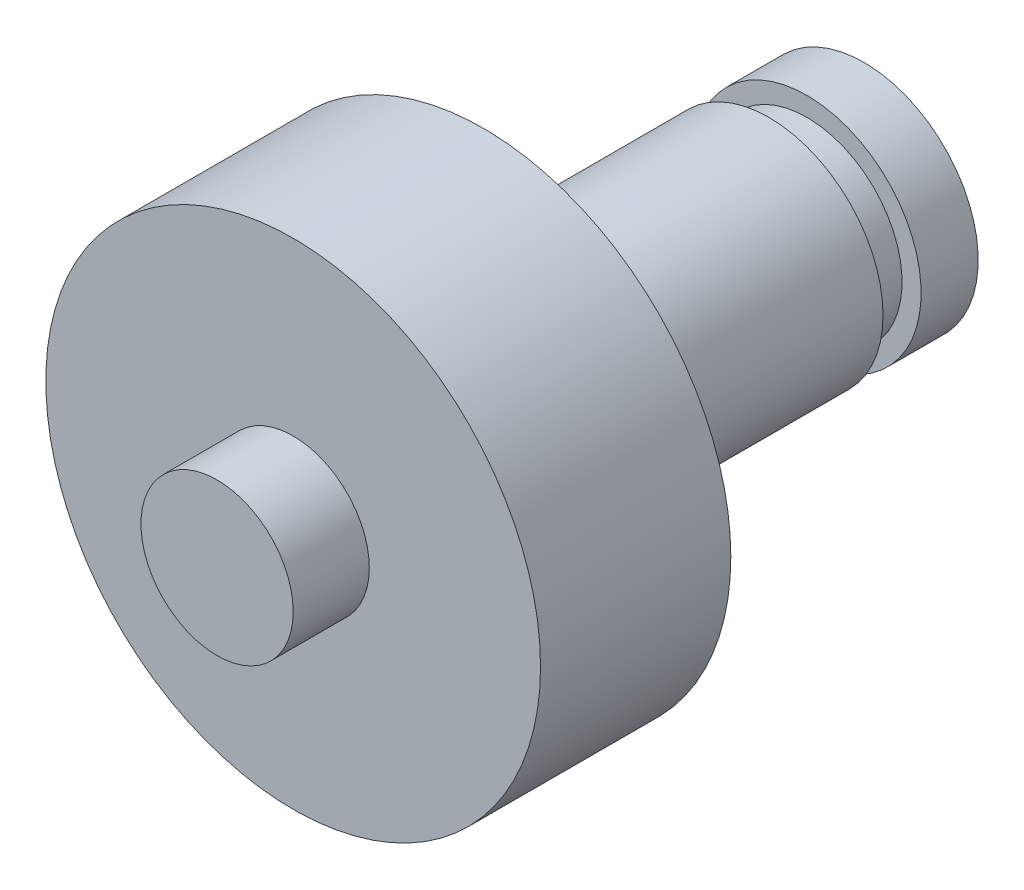
from build123d import *

# Parameters (mm, degrees)
SKETCH1_R      = 6.5
EXTRUDE1_DEPTH = 5
SKETCH2_R      = 2
EXTRUDE2_DEPTH = 2
SKETCH3_R      = 3
EXTRUDE3_DEPTH = 7.5
SKETCH4_R      = 2.5
EXTRUDE5_DEPTH = 1
SKETCH6_R      = 3
EXTRUDE6_DEPTH = 1.5


with BuildPart() as part:
    # Sketch1 → Extrude1 (new body)
    with BuildSketch(Plane.XY):
        Circle(SKETCH1_R)
    extrude(amount=EXTRUDE1_DEPTH)

    # Sketch2 → Extrude2 (add)
    with BuildSketch(Plane.XY.offset(5)):
        Circle(SKETCH2_R)
    extrude(amount=EXTRUDE2_DEPTH)

    # Sketch3 → Extrude3 (add)
    with BuildSketch(Plane(origin=(0, 0, 0), x_dir=(-1, 0, 0), z_dir=(0, 0, -1))):
        with Locations(Location((0, 0, 0), (0, 0, 180))):
            Circle(SKETCH3_R)
    extrude(amount=EXTRUDE3_DEPTH)

    # Sketch4 → Extrude5 (add)
    with BuildSketch(Plane(origin=(0, 0, -7.5), x_dir=(-1, 0, 0), z_dir=(0, 0, -1))):
        Circle(SKETCH4_R)
    extrude(amount=EXTRUDE5_DEPTH)

    # Sketch6 → Extrude6 (add)
    with BuildSketch(Plane(origin=(0, 0, -8.5), x_dir=(-1, 0, 0), z_dir=(0, 0, -1))):
        with Locations(Location((0, 0, 0), (0, 0, 180))):
            Circle(SKETCH6_R)
    extrude(amount=EXTRUDE6_DEPTH)


solid = part.part
